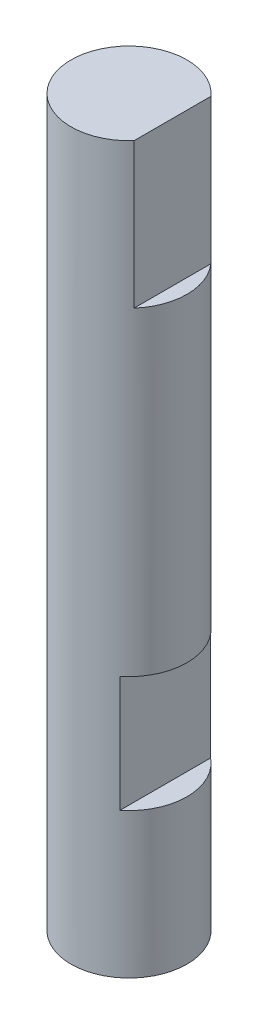
from build123d import *

# Parameters (mm, degrees)
SKETCH1_R               = 8
BOSS_EXTRUDE1_DEPTH     = 100
CUT_EXTRUDE1_DEPTH      = 101.637965003
CUT_EXTRUDE1_DEPTH_BACK = 101.637965003
SKETCH2_W               = 2
SKETCH2_H               = 20
SKETCH2_W_2             = 6
SKETCH2_H_2             = 16


with BuildPart() as part:
    # Sketch1 → Boss-Extrude1 (new body)
    with BuildSketch(Plane(origin=(0, 0, 0), x_dir=(1, 0, 0), z_dir=(0, 1, 0))):
        with Locations(Location((0, 0, 0), (0, 0, 270))):
            Circle(SKETCH1_R)
    extrude(amount=BOSS_EXTRUDE1_DEPTH)

    # Sketch2 → Cut-Extrude1 (cut, two sides: drawn at the far end of the back side and taken through both)
    with BuildSketch(Plane.XY.offset(-CUT_EXTRUDE1_DEPTH_BACK)):
        with Locations((7, 90)):
            Rectangle(SKETCH2_W, SKETCH2_H)
        with Locations((8, 28)):
            Rectangle(SKETCH2_W_2, SKETCH2_H_2)
    extrude(amount=CUT_EXTRUDE1_DEPTH + CUT_EXTRUDE1_DEPTH_BACK, mode=Mode.SUBTRACT)


solid = part.part
